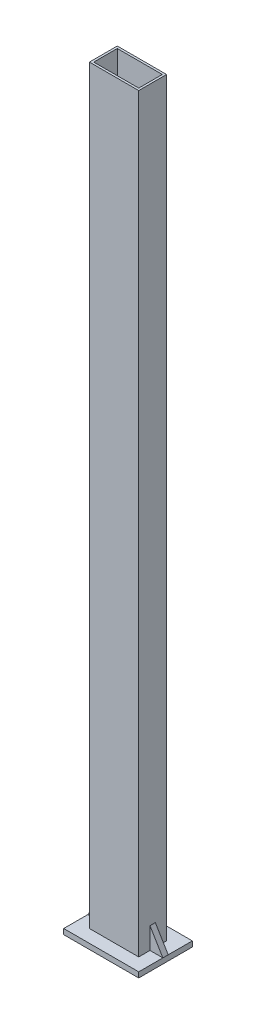
from build123d import *

# Parameters (mm, degrees)
SKETCH2_W           = 70
SKETCH2_H           = 50
BOSS_EXTRUDE1_DEPTH = 5
SKETCH3_W           = 46
SKETCH3_H           = 26
BOSS_EXTRUDE2_DEPTH = 700
BOSS_EXTRUDE3_DEPTH = 2.5
SKETCH5_W           = 42
SKETCH5_H           = 22
CUT_EXTRUDE1_DEPTH  = 691


with BuildPart() as part:
    # Sketch2 → Boss-Extrude1 (new body)
    with BuildSketch(Plane(origin=(0, 0, 0), x_dir=(1, 0, 0), z_dir=(0, 1, 0))):
        with Locations((-450, 0)):
            Rectangle(SKETCH2_W, SKETCH2_H)
    extrude(amount=BOSS_EXTRUDE1_DEPTH)

    # Sketch3 → Boss-Extrude2 (add)
    with BuildSketch(Plane(origin=(0, 5, 0), x_dir=(1, 0, 0), z_dir=(0, 1, 0))):
        with Locations((-450, 0)):
            Rectangle(SKETCH3_W, SKETCH3_H)
    extrude(amount=BOSS_EXTRUDE2_DEPTH)

    # Sketch4 → Boss-Extrude3 (add, symmetric)
    with BuildSketch(Plane.XY):
        Polygon((-473, 5), (-485, 5), (-473, 25), align=None)
        Polygon((-427, 25), (-427, 5), (-415, 5), align=None)
    extrude(amount=BOSS_EXTRUDE3_DEPTH, both=True)

    # Sketch5 → Cut-Extrude1 (cut)
    with BuildSketch(Plane(origin=(0, 705, 0), x_dir=(1, 0, 0), z_dir=(0, 1, 0))):
        with Locations((-450, 0)):
            Rectangle(SKETCH5_W, SKETCH5_H)
    extrude(amount=-CUT_EXTRUDE1_DEPTH, mode=Mode.SUBTRACT)


solid = part.part
